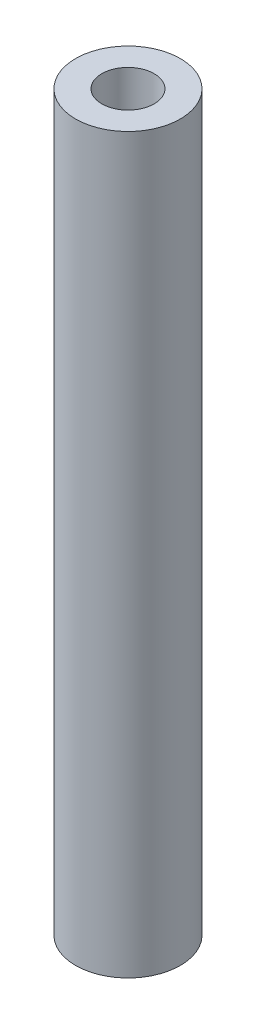
SolidWorks part; units mm, degrees
ref_plane "Front Plane" through (0, 0, 0) normal (0, 0, 1) x (1, 0, 0)
ref_plane "Top Plane" through (0, 0, 0) normal (0, 1, 0) x (1, 0, 0)
ref_plane "Right Plane" through (0, 0, 0) normal (1, 0, 0) x (0, 0, -1)
sketch "Sketch1" plane through (0, 0, 0) normal (0, 1, 0) x (1, 0, 0)
  circle A0 centre (0, 0) radius 20
  circle A1 centre (0, 0) radius 10
  dimension "D1" = 40
  dimension "D2" = 20
extrude "Boss-Extrude1" add sketch "Sketch1" along normal mid plane 280
